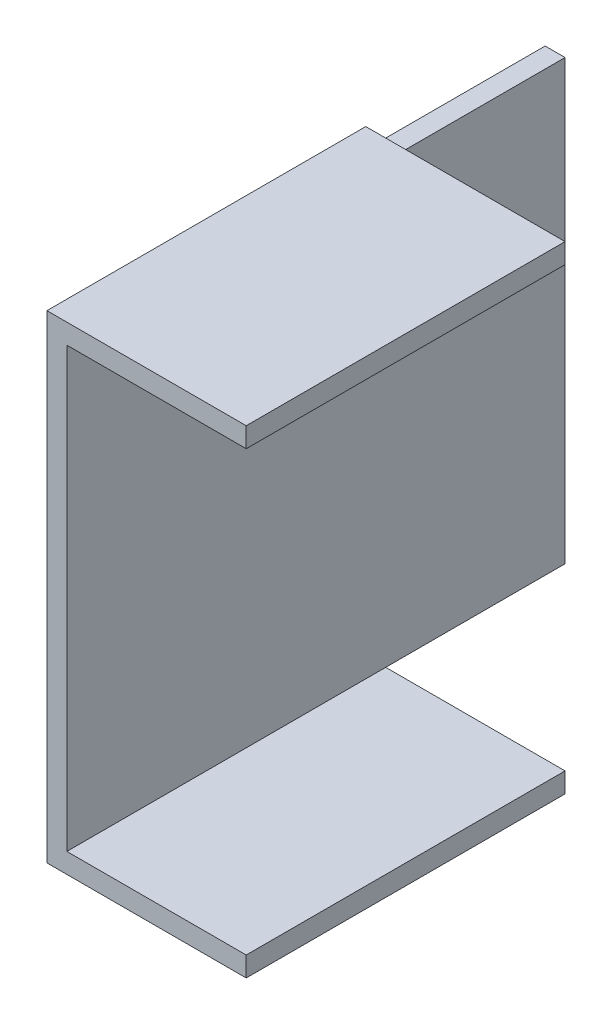
SolidWorks part; units mm, degrees
ref_plane "前视基准面" through (0, 0, 0) normal (0, 0, 1) x (1, 0, 0)
ref_plane "上视基准面" through (0, 0, 0) normal (0, 1, 0) x (1, 0, 0)
ref_plane "右视基准面" through (0, 0, 0) normal (1, 0, 0) x (0, 0, -1)
sketch "草图1" plane through (0, 0, 0) normal (0, 0, 1) x (1, 0, 0)
  line L0 (0, 0) -> (0, 120)
  line L1 (0, 120) -> (50, 120)
  line L2 (0, 0) -> (50, 0)
  line L3 (5, 5) -> (50, 5)
  line L4 (5, 5) -> (5, 115)
  line L5 (5, 115) -> (50, 115)
  line L6 (50, 115) -> (50, 120)
  line L7 (50, 0) -> (50, 5)
  dimension "D1" = 5
extrude "凸台-拉伸1" add sketch "草图1" against normal blind 150
sketch "草图2" plane through (0, 0, -150) normal (0, 0, -1) x (-1, 0, 0)
  line L0 (-50, 120) -> (0, 120)
  line L1 (0, 120) -> (0, 115)
  line L2 (0, 120) -> (0, 0) construction
  line L3 (0, 115) -> (-50, 115)
  line L4 (-50, 115) -> (-50, 120)
  line L5 (-50, 0) -> (-50, 5)
  line L6 (-50, 5) -> (0, 5)
  line L7 (0, 5) -> (0, 0)
  line L8 (0, 0) -> (-50, 0)
extrude "切除-拉伸1" cut sketch "草图2" against normal blind 45
sketch "草图3" plane through (0, 0, -150) normal (0, 0, -1) x (-1, 0, 0)
  line L8 (-5, 115) -> (-5, 5)
  line L9 (-5, 5) -> (0, 5)
  line L10 (0, 5) -> (0, 115)
  line L11 (0, 115) -> (-5, 115)
  line L12 (-5, 115) -> (-5, 5)
  line L13 (-5, 5) -> (0, 5)
  line L14 (0, 5) -> (0, 115)
  line L15 (0, 115) -> (-5, 115)
  dimension "D1" = 0
extrude "切除-拉伸2" cut sketch "草图3" against normal blind 25
sketch "草图4" plane through (0, 0, -105) normal (0, 0, -1) x (-1, 0, 0)
  line L10 (-50, 0) -> (0, 0)
  line L11 (0, 0) -> (0, 5)
  line L12 (0, 5) -> (-5, 5)
  line L13 (-5, 5) -> (-50, 5)
  line L14 (-50, 5) -> (-50, 0)
  line L15 (-50, 0) -> (0, 0)
  line L16 (0, 0) -> (0, 5)
  line L17 (0, 5) -> (-5, 5)
  line L18 (-5, 5) -> (-50, 5)
  line L19 (-50, 5) -> (-50, 0)
  dimension "D1" = 0
extrude "切除-拉伸3" cut sketch "草图4" against normal blind 25
sketch "草图5" plane through (0, 0, -105) normal (0, 0, -1) x (-1, 0, 0)
  line L10 (-50, 120) -> (-50, 115)
  line L11 (-50, 115) -> (-5, 115)
  line L12 (-5, 115) -> (0, 115)
  line L13 (0, 115) -> (0, 120)
  line L14 (0, 120) -> (-50, 120)
  line L15 (-50, 120) -> (-50, 115)
  line L16 (-50, 115) -> (-5, 115)
  line L17 (-5, 115) -> (0, 115)
  line L18 (0, 115) -> (0, 120)
  line L19 (0, 120) -> (-50, 120)
  dimension "D1" = 0
extrude "切除-拉伸4" cut sketch "草图5" against normal blind 25
